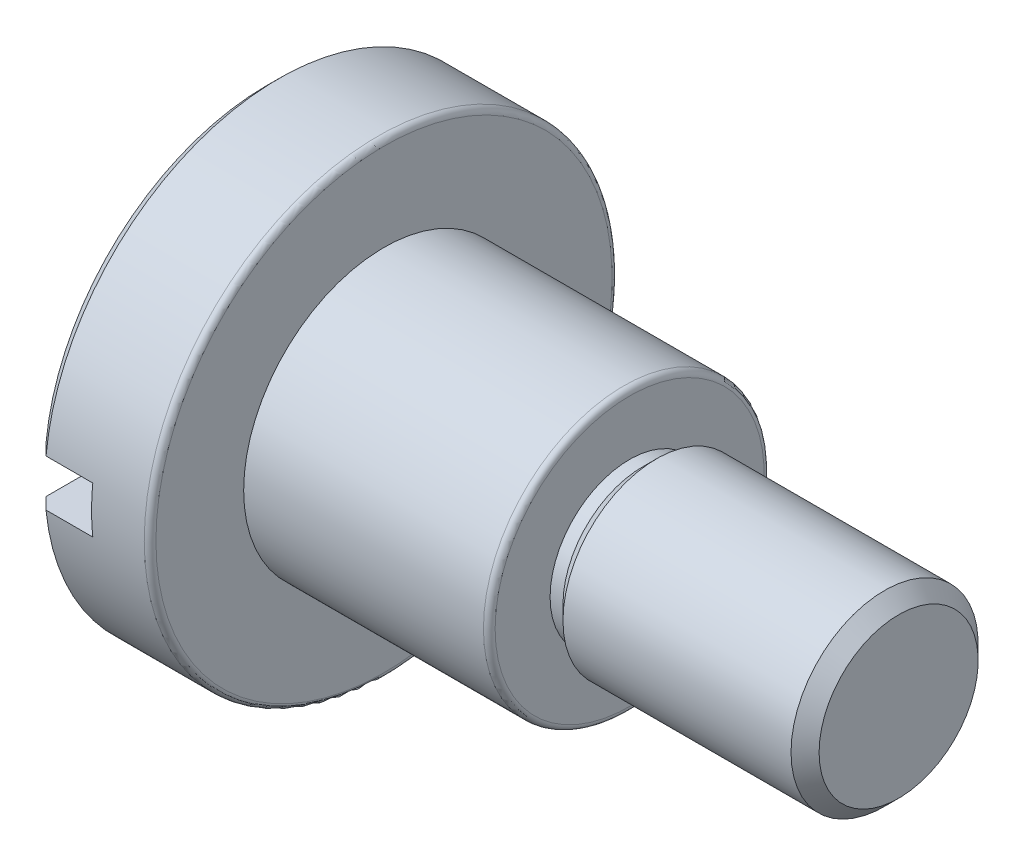
from build123d import *

# Parameters (mm, degrees)
CHAMFER1_SIZE           = 0.5
CUT_EXTRUDE1_DEPTH      = 31.479501308
CUT_EXTRUDE1_DEPTH_BACK = 31.479501308
SKETCH3_W               = 2.5
SKETCH3_H               = 2
FILLET1_R               = 0.25


with BuildPart() as part:
    # Sketch2 → Revolve1 (revolve)
    with BuildSketch(Plane.XY, mode=Mode.PRIVATE) as revolve1_sk:
        Polygon((0, 0), (0, 10), (5, 10), (5, 6), (15.5, 6), (15.5, 4), (15.5, 3.4), (16.05, 3.4), (16.65, 4), (26.4, 4), (27, 3.4), (27, 0), align=None)
    revolve(revolve1_sk.sketch.rotate(Axis((0, 0, 0), (1, 0, 0)), 90), axis=Axis((0, 0, 0), (1, 0, 0)))

    # Chamfer1
    chamfer1_edges = [part.edges().sort_by_distance(p)[0] for p in [
        (0, 0, -10),
    ]]
    chamfer(chamfer1_edges, length=CHAMFER1_SIZE)

    # Sketch3 → Cut-Extrude1 (cut, two sides: drawn at the far end of the back side and taken through both)
    with BuildSketch(Plane.XY.offset(-CUT_EXTRUDE1_DEPTH_BACK)):
        with Locations((1.25, 0)):
            Rectangle(SKETCH3_W, SKETCH3_H)
    extrude(amount=CUT_EXTRUDE1_DEPTH + CUT_EXTRUDE1_DEPTH_BACK, mode=Mode.SUBTRACT)

    # Fillet1
    fillet1_edges = [part.edges().sort_by_distance(p)[0] for p in [
        (15.5, 0, -6),
        (5, 0, -10),
    ]]
    fillet(fillet1_edges, radius=FILLET1_R)


solid = part.part
